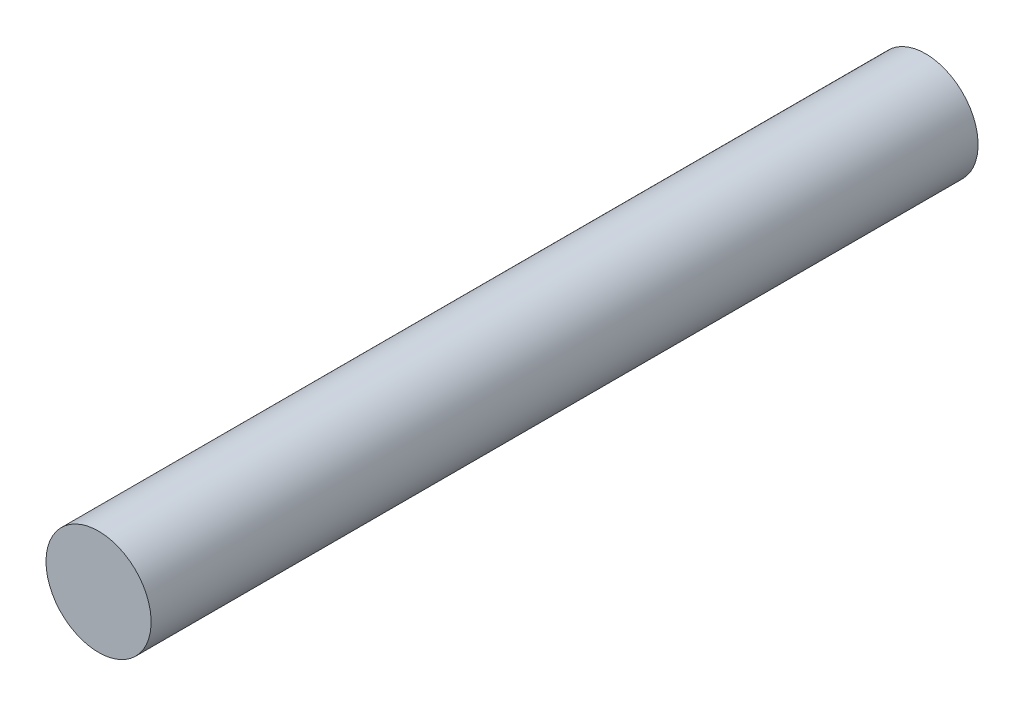
from build123d import *

# Parameters (mm, degrees)
SKETCH_1_R      = 15
EXTRUDE_1_DEPTH = 236


with BuildPart() as part:
    # 草图1 → 凸台-拉伸1 (new body)
    with BuildSketch(Plane.XY):
        with Locations(Location((0, 0, 0), (0, 0, 180))):
            Circle(SKETCH_1_R)
    extrude(amount=EXTRUDE_1_DEPTH)


solid = part.part
